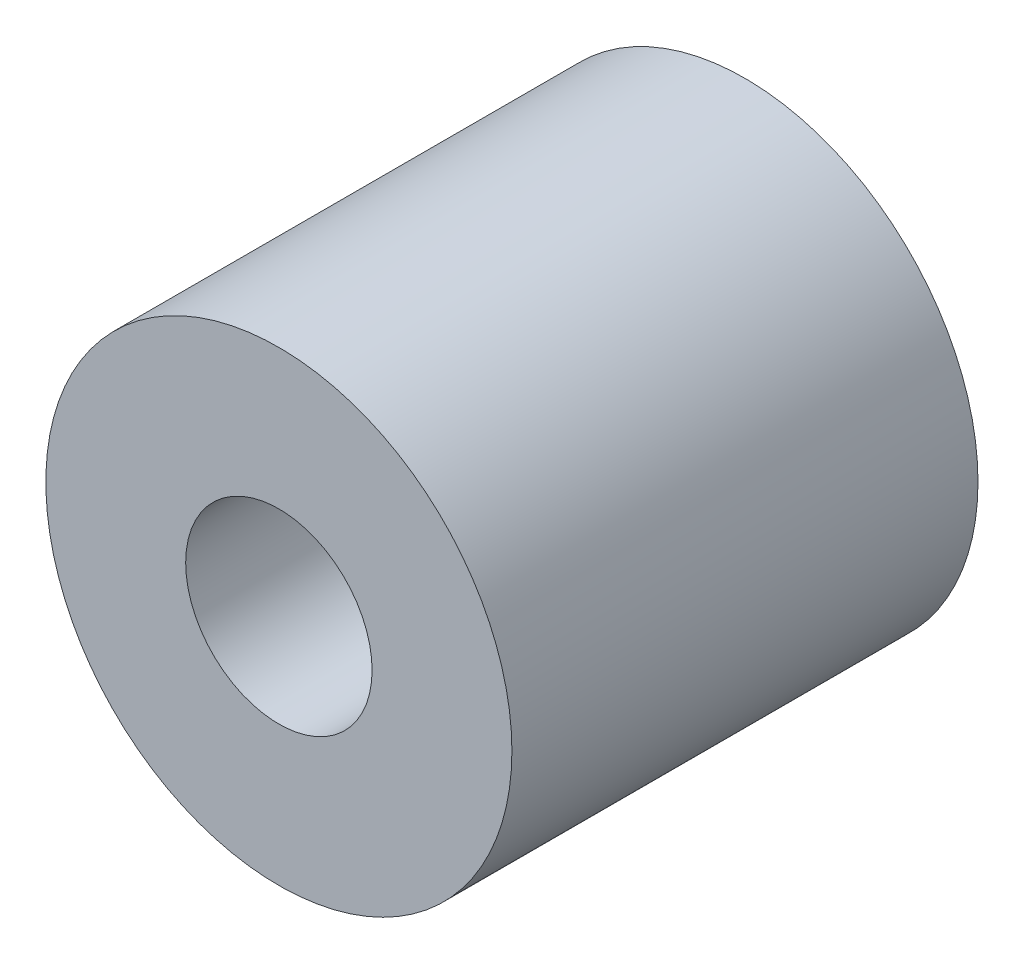
SolidWorks part; units mm, degrees
ref_plane "前视基准面" through (0, 0, 0) normal (0, 0, 1) x (1, 0, 0)
ref_plane "上视基准面" through (0, 0, 0) normal (0, 1, 0) x (1, 0, 0)
ref_plane "右视基准面" through (0, 0, 0) normal (1, 0, 0) x (0, 0, -1)
other "Configuration Table"
sketch "草图1" plane through (0, 0, 0) normal (0, 0, 1) x (1, 0, 0)
  circle A0 centre (0, 0) radius 4
  circle A1 centre (0, 0) radius 10
extrude "凸台-拉伸1" add sketch "草图1" along normal blind 20
